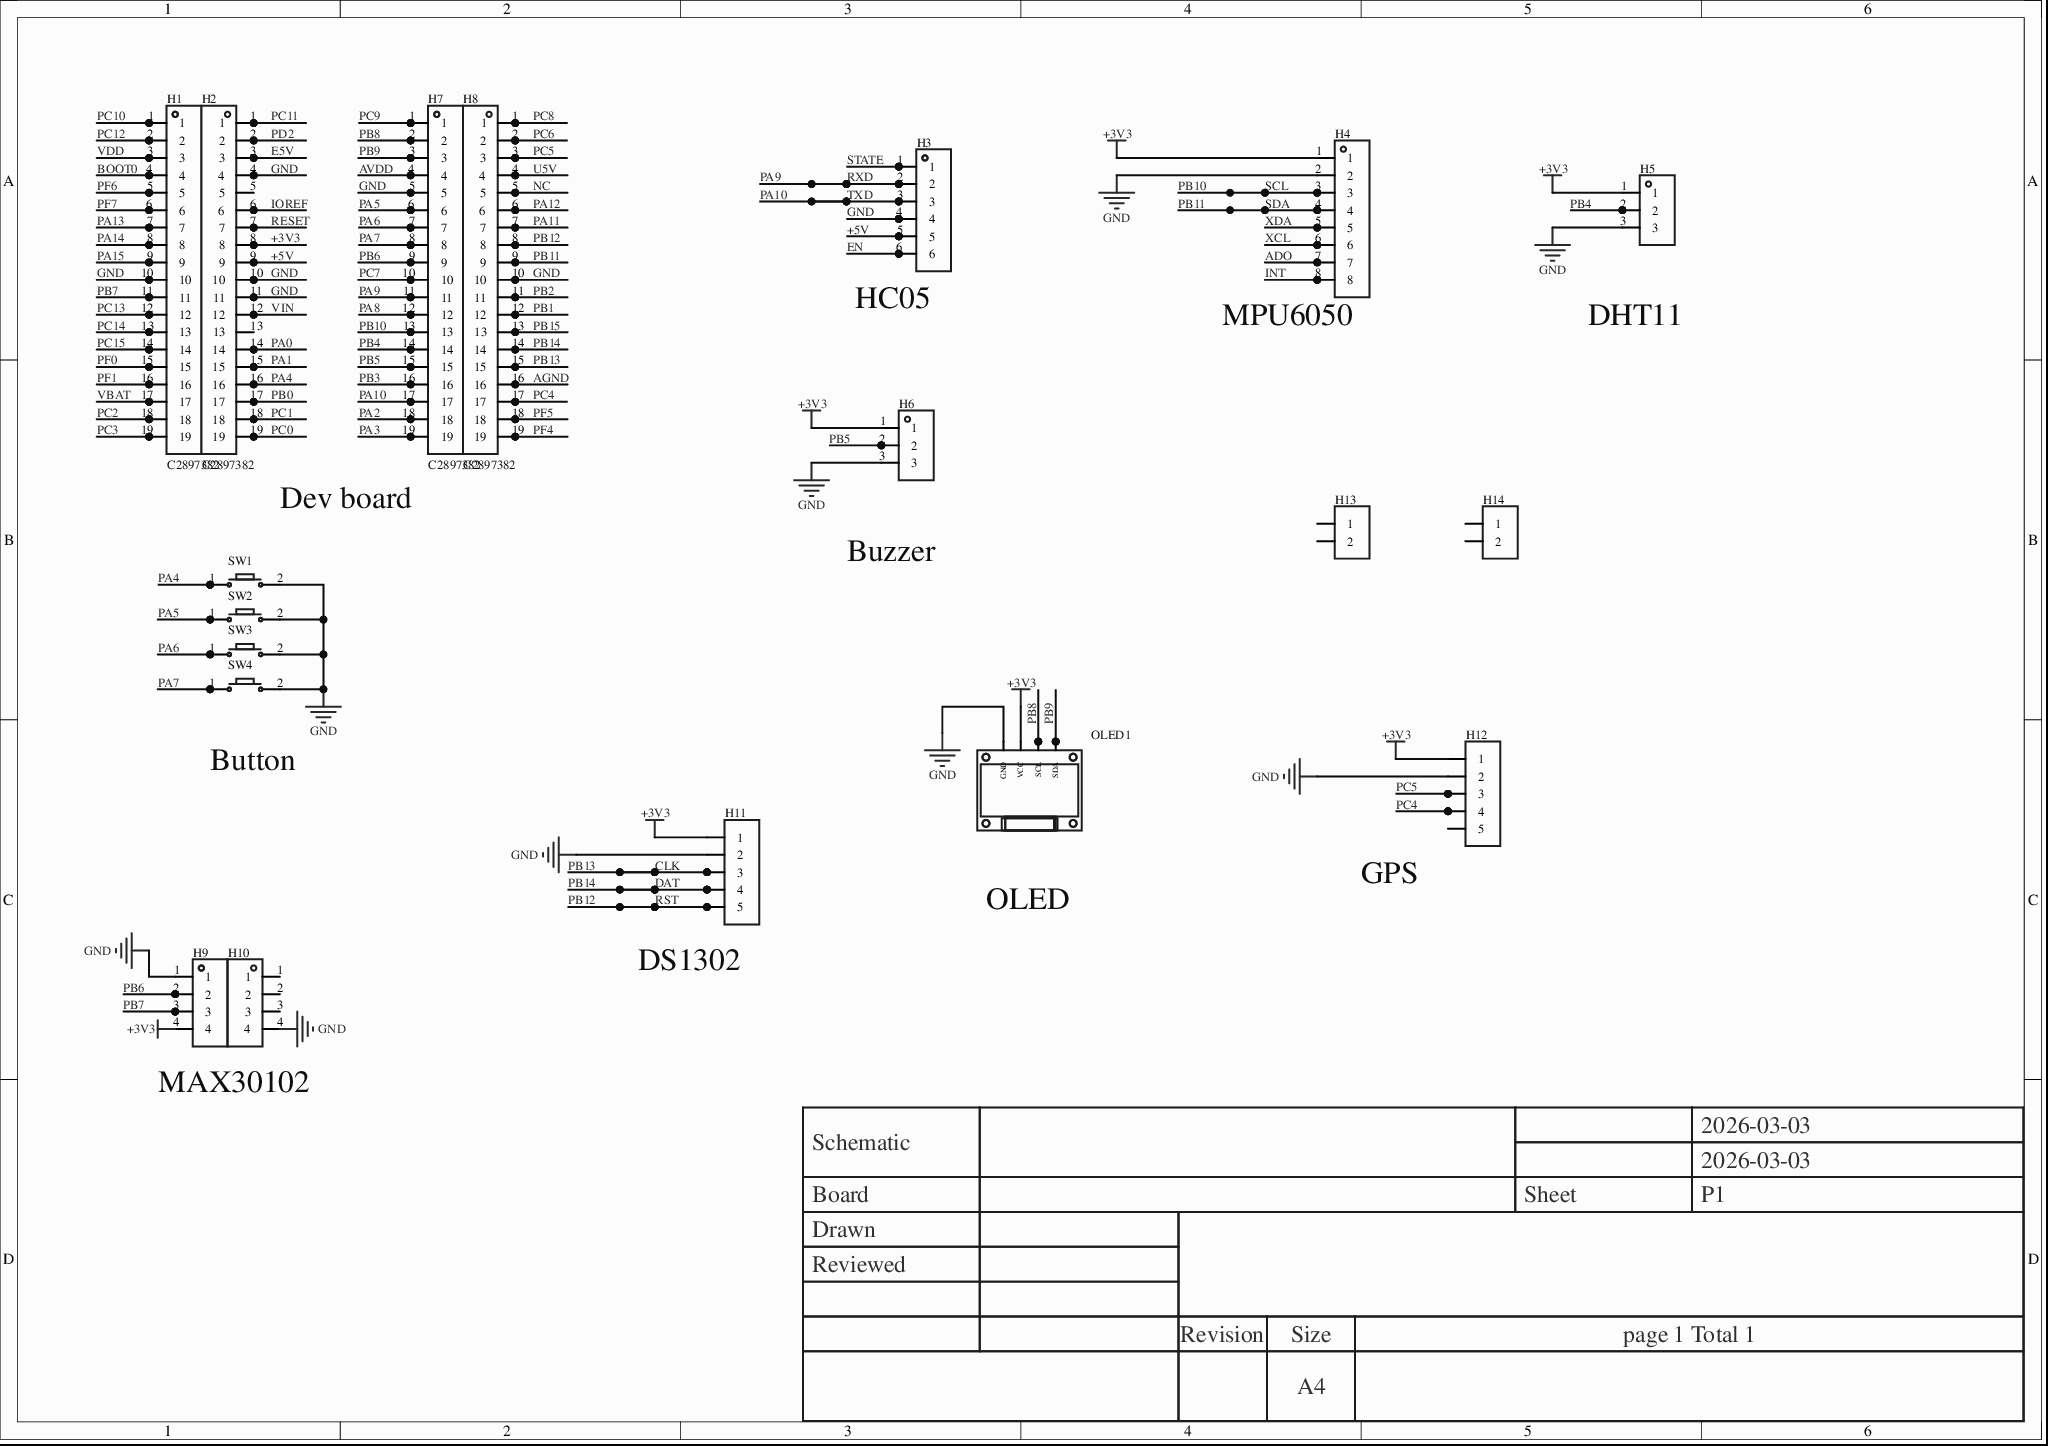
[diagram p0: MISC49932-3.schdoc]
# Altium project MISC49932-2.PrjPcb
1 sheet, 19 parts. Net scope: global (net labels, ports and power ports of the same name join across sheets).
Board file: MISC49932.pcbdoc

## Sheet MISC49932-3.schdoc
size 297 x 209 mm; Version: V1.0; @Project Name: MISC49932; @Update Date: 2026-03-27; @Create Date: 2026-03-27; @Board Name: MISC49932; @Create Time: 16:08:49; @Page Count: 1; @Page No: 1; @Schematic Name: MISC49932; @Update Time: 16:08:49; Size: A4

### Parts
H1  C2897382  [HDR-TH_19P-P2.54-V-F]
H2  C2897382  [HDR-TH_19P-P2.54-V-F]
H3  (no value)  [HDR-TH_6P-P2.54-V-F]
H4  (no value)  [HDR-TH_8P-P2.54-V-F-1]
H5  (no value)  [HDR-TH_3P-P2.54-V-F]
H6  (no value)  [HDR-TH_3P-P2.54-V-F]
H7  C2897382  [HDR-TH_19P-P2.54-V-F]
H8  C2897382  [HDR-TH_19P-P2.54-V-F]
H9  (no value)  [HDR-TH_4P-P2.54-V-F]
H10  (no value)  [HDR-TH_4P-P2.54-V-F]
H11  (no value)  [HDR-TH_5P-P2.54-V-F]
H12  (no value)  [HDR-TH_5P-P2.54-V-F]
H13  (no value)  [HDR-TH_2P-P2.54-V-F]
H14  (no value)  [HDR-TH_2P-P2.54-V-F]
OLED1  (no value)  [0.96OLED_4P]
SW1  (no value)  [Key_SMD_3.6x6.1x2.5]
SW2  (no value)  [Key_SMD_3.6x6.1x2.5]
SW3  (no value)  [Key_SMD_3.6x6.1x2.5]
SW4  (no value)  [Key_SMD_3.6x6.1x2.5]

### Nets
+3V3: H2.8 H4.1 H5.1 H6.1 H9.4 H11.1 H12.1 OLED1.2(VCC)
GND: H1.10 H2.4 H2.10 H2.11 H3.4 H4.2 H5.3 H6.3 H7.5 H8.10 H9.1 H10.4 H11.2 H12.2 OLED1.1(GND) SW1.2 SW2.2 SW3.2 SW4.2
+5V: H2.9 H3.5
ADO: H4.7
AGND: H8.16
AVDD: H7.4
BOOT0: H1.4
CLK: H8.15 H11.3  [also labelled PB13]
DAT: H8.14 H11.4  [also labelled PB14]
E5V: H2.3
EN: H3.6
INT: H4.8
IOREF: H2.6
NC: H8.5
PA0: H2.14
PA1: H2.15
PA2: H7.18
PA3: H7.19
PA4: H2.16 SW1.1
PA5: H7.6 SW2.1
PA6: H7.7 SW3.1
PA7: H7.8 SW4.1
PA8: H7.12
PA9: H3.2 H7.11  [also labelled RXD]
PA10: H3.3 H7.17  [also labelled TXD]
PA11: H8.7
PA12: H8.6
PA13: H1.7
PA14: H1.8
PA15: H1.9
PB0: H2.17
PB1: H8.12
PB2: H8.11
PB3: H7.16
PB4: H5.2 H7.14
PB5: H6.2 H7.15
PB6: H7.9 H9.2
PB7: H1.11 H9.3
PB8: H7.2 OLED1.3(SCL)
PB9: H7.3 OLED1.4(SDA)
PB10: H4.3 H7.13  [also labelled SCL]
PB11: H4.4 H8.9  [also labelled SDA]
PB12: H8.8 H11.5  [also labelled RST]
PB15: H8.13
PC0: H2.19
PC1: H2.18
PC2: H1.18
PC3: H1.19
PC4: H8.17 H12.4
PC5: H8.3 H12.3
PC6: H8.2
PC7: H7.10
PC8: H8.1
PC9: H7.1
PC10: H1.1
PC11: H2.1
PC12: H1.2
PC13: H1.12
PC14: H1.13
PC15: H1.14
PD2: H2.2
PF0: H1.15
PF1: H1.16
PF4: H8.19
PF5: H8.18
PF6: H1.5
PF7: H1.6
RESET: H2.7
STATE: H3.1
U5V: H8.4
VBAT: H1.17
VDD: H1.3
VIN: H2.12
XCL: H4.6
XDA: H4.5

Not connected (* = marked no-connect by the designer): H2 5 13; H10 1 2 3; H12 5; H13 1 2; H14 1 2

### Notes on the sheet
- (near H3) HC05
- (near H4) MPU6050
- DHT11
- Dev board
- Buzzer
- (near SW4) Button
- OLED
- (near H12) GPS
- (near H11) DS1302
- MAX30102
- 2026-03-03
- Schematic
- Board
- Sheet
- P1
- Drawn
- Reviewed
- Revision
- Size
- A4
- page 1 Total 1

### Library data of the parts
H1 H2 H7 H8 = HDR-F_2.54_1x19P: ConvertToPcb: yes; ModelId: 131ee080550a465daf9368d356f53fe90819f05c4eef4c71ace90d822a990e87; ModelName: HDR-TH_19P-P2.54-F-LI-1X19P; ModelTransform: 1919.68128,95.6691,0,0,0,0,0,0,-125.984; Device: HDR-F_2.54_1x19P; Symbol: HDR-F_2.54_1x19P; FootprintName: HDR-TH_19P-P2.54-V-F; AddInBom: yes; Supplier Footprint: 插件; ManufacturerPart: C2897382
H3 = HDR-F_2.54_1x6P: Symbol: Header-Female-2.54_1x6; ConvertToPcb: yes; ModelId: 0f5bcf94dcda47d085f24cdca1696fe90819f05c4eef4c71ace90d822a990e87; ModelTransform: 619.684,94.488,0,0,0,0,0,0,-125.984; Device: HDR-F_2.54_1x6P; FootprintName: HDR-TH_6P-P2.54-V-F; AddInBom: yes; SupplierPart: C40877; Supplier Footprint: 插件; ModelName: HDR-TH_6P-P2.54-V-F
H4 = HDR-F_2.54_1x8P: Symbol: Header-Female-2.54_1x8; AddInBom: yes; ModelId: 0f7e4d9227ef4fa08d5469c22cc70cdb0819f05c4eef4c71ace90d822a990e87; ModelName: HDR-F-2.54_1x8; ModelTransform: 799.99844,100,0,0,0,0,0,0,-118.11; Device: HDR-F_2.54_1x8P; FootprintName: HDR-TH_8P-P2.54-V-F-1; ConvertToPcb: yes; SupplierPart: C27438; Supplier Footprint: 插件
H5 H6 = HDR-F_2.54_1x3P: Symbol: PM254V-11-03-H85; ConvertToPcb: yes; ModelId: f3b3cc5aae9641bf9e56fc160cef875b0819f05c4eef4c71ace90d822a990e87; ModelName: HDR2.54-F-LI-1X3P; ModelTransform: 299.9994,100,0,0,0,0,0,0,-118.11; Device: HDR-F_2.54_1x3P; FootprintName: HDR-TH_3P-P2.54-V-F; AddInBom: yes; SupplierPart: C541850; Supplier Footprint: 插件
H9 H10 = HDR-F_2.54_1x4P: Symbol: 2.54-1*4P female; ConvertToPcb: yes; ModelId: d187812051054f85879fcaa51a310d8e0819f05c4eef4c71ace90d822a990e87; ModelTransform: 419.6842,98.464,0,0,0,0,0,0,-118.11; Device: HDR-F_2.54_1x4P; FootprintName: HDR-TH_4P-P2.54-V-F; AddInBom: yes; SupplierPart: C2718488; Supplier Footprint: 插件; ModelName: HDR-TH_4P-P2.54-V-F
H11 = HDR-F_2.54_1x5P: Symbol: Header-Female-2.54_1x5; ConvertToPcb: yes; ModelId: f49cb6116a3d45e5a64915bf3e00773f0819f05c4eef4c71ace90d822a990e87; ModelTransform: 519.684,98.464,0,0,0,0,0,0,-124.016; Device: HDR-F_2.54_1x5P; FootprintName: HDR-TH_5P-P2.54-V-F; AddInBom: yes; SupplierPart: C50950; Supplier Footprint: 插件; ModelName: HDR-TH_5P-P2.54-V-F
H12 = HDR-F_2.54_1x5P: Symbol: Header-Female-2.54_1x5; 3D Model: f49cb6116a3d45e5a64915bf3e00773f0819f05c4eef4c71ace90d822a990e87; 3D Model Transform: 519.684,98.464,0,0,0,0,0,0,-124.016; ConvertToPcb: yes; Device: HDR-F_2.54_1x5P; Supplier Part: C50950; Supplier Footprint: 插件; FootprintName: HDR-TH_5P-P2.54-V-F; AddInBom: yes; ModelName: HDR-TH_5P-P2.54-V-F
H13 H14 = HDR-F_2.54_1x2P: Symbol: Header-Female-2.54_1x2; ConvertToPcb: yes; ModelId: a9450ef445564560a104363b9aacde4e0819f05c4eef4c71ace90d822a990e87; ModelName: HDR-TH_2P-P2.54-F-LI-1X2P; ModelTransform: 215.7476,98.425,0,0,0,0,0,0,-129.921; Device: HDR-F_2.54_1x2P; FootprintName: HDR-TH_2P-P2.54-V-F; AddInBom: yes; SupplierPart: C49661; Supplier Footprint: 插件
OLED1 = 0.96OLED模块_4P: Device: 0.96OLED module_4P; ConvertToPcb: yes; ModelId: 79c000fdb68d45a296c2e9bedf4f90550819f05c4eef4c71ace90d822a990e87; ModelTransform: 1393.69792,1318.895,0,0,0,0,0,-560.079,-137.795; Symbol: 0.96OLED module_4P; FootprintName: 0.96OLED_4P; AddInBom: yes; Supplier Footprint: 插件; ModelName: 0.96OLED_4P
SW1-SW4 = Key_SMD_3.6x6.1x2.5: Symbol: Tact switch x2; AddInBom: yes; ModelId: 90d18ad19a7e424ebd3215e1b5dcb80c0819f05c4eef4c71ace90d822a990e87; ModelName: KEY-SMD_2P-L6.0-W3.6-H2.5-LS8.0 COPY; ModelTransform: 311.02,141.73,102.36,0,0,0,0,0,0; Device: Key_SMD_3.6x6.1x2.5; FootprintName: Key_SMD_3.6x6.1x2.5; ConvertToPcb: yes; Supplier Footprint: SMD